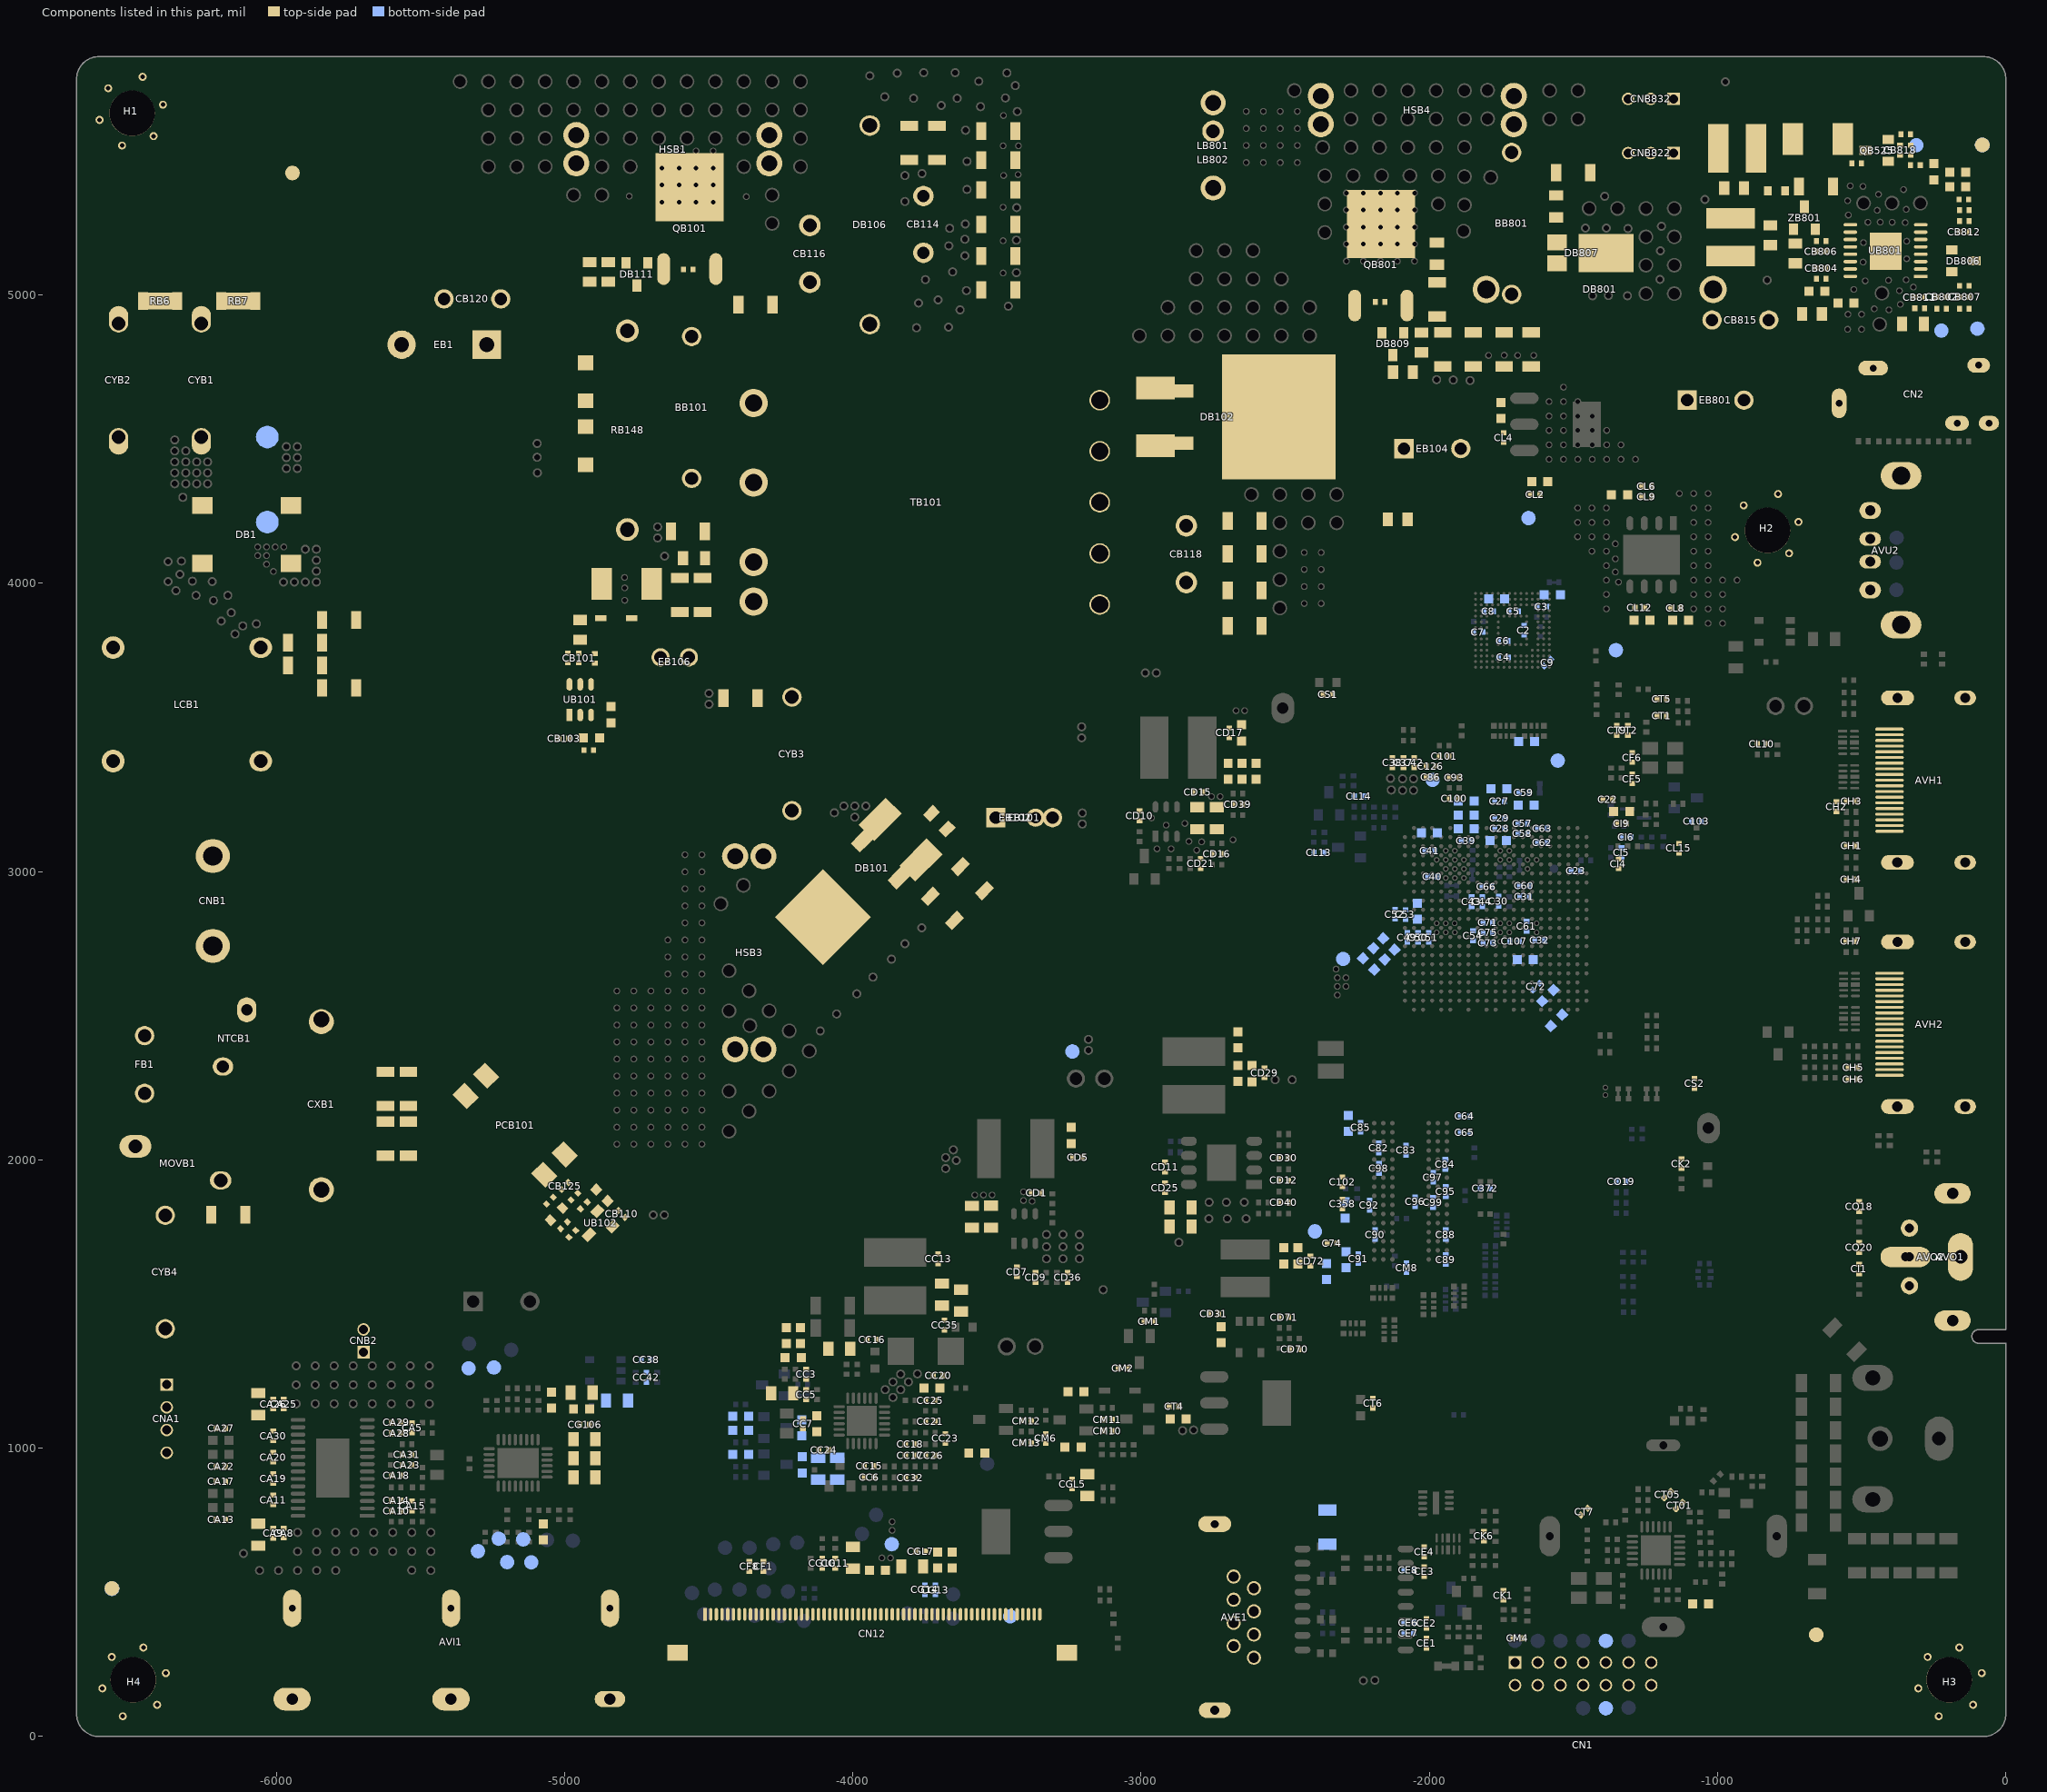
[diagram p0: the components of this part, seen from the top]
# Altium PCB MISC84395.PcbDoc (part 2 of 26)
Units mil, origin at the board's own origin, x right, y up, seen from the top; angles counter-clockwise.
Board outline 6692.91 x 5826.77 mil, 2 copper layers (TopLayer, BottomLayer), stack 61.855 mil thick; 951 components, 565 nets, 4374 pads, 1804 vias.
Unrouted connection lines stored in the file: 1.

## Classes and differential pairs (continued)
component class PS#01_XXXXXXXXXXXXXXXX: ADIM BB101 BB801 BL_ON CB101 CB102 CB103 CB109 CB110 CB111 CB113 CB114 CB116 CB117 CB118 CB120 CB125 CB802 CB803 CB804 CB805 CB806 CB807 CB809 CB810 CB811 CB812 CB813 CB814 CB815 CB816 CB818 CB819 CNB1 CNB2 CNB822 CNB832 "Conformal Coating" CXB1 CXB2 CYB1 CYB2 CYB3 CYB4 DB1 DB101 DB102 DB104 DB106 DB109 DB110 DB111 DB121 DB801 DB802 DB806 DB807 DB809 EB1 EB101 EB102 EB104 EB106 EB801 EVA1 EVA2 EVA3 EVA4 EVA5 EVA6 FB1 GD1 GD2 GD3 GD4 GL1 GL2 HSB1 HSB3 HSB4 LB801 LB802 LB804 LB805 LCB1 LCB2 ML1 MOVB1 NTCB1 PCB101 PWM_DIM QB101 QB525 QB801 RB1 RB2 RB3 RB4 RB5 RB6 RB7 RB101 RB102 RB103 RB104 RB105 RB106 RB107 RB109 RB114 RB115 RB116 RB117 RB118 RB119 RB121 RB124 RB125 RB126 RB128 RB129 RB130 RB131 RB132 RB133 RB134 RB135 RB136 RB140 RB141 RB142 RB148 RB151 RB152 RB153 RB154 RB155 RB156 RB158 RB801 RB802 RB803 RB804 RB805 RB806 RB807 RB808 RB809 RB810 RB811 RB812 RB814 RB816 RB818 RB819 RB820 RB821 RB822 RB824 RB825 RB826 RB827 RB830 RB832 RB833 RB834 RB837 TB101 TP-TDT UB101 UB102 UB801 ZB801
component class PCB_info: AI_V CAUTION COLD CQC H1 H2 H3 H4 "High Voltage" HOT M1 M2 M3 M4 M5 M6 MAC Manufacture_Info S/N1 S/N2
polygon class Poly_5mil: 5 5mil
pad class HS60: Free-HS60
pad class VIA5: Free-VIA5

## Components (designator, comment, footprint, x,y, rotation, side; value= is the part's Value field where it differs from the comment)
1V8_M "TEST" TP#1 -1554.58,3384.95 r270 bottom
3V3_M "TEST" TP#1 -1352.83,3768 r180 bottom
3V3_STB "TEST" TP#1 -1656,4226 r90 bottom
5V_STB "TEST" TP#2 -3238.17,2376 r90 bottom
5V_WIFI "TEST" TP#2 -1387.74,98 r90 bottom
+1.5V_DDR "TEST" TP#1 -2397,1752 r90 bottom
+1.05V_VDDC_CPU "TEST" TP#1 -2299,2697 r270 bottom
+1.10V_VDDC "TEST" TP#1 -1989,3318 r270 bottom
ADIM "NC/TEST" TP_BL -311,5519 r270 bottom
AI_V "AI_GRIPPER_V" AI_GRIPPER_V 6418,1068.5 r90 top
AVDD "TEST" TP#1 -3865,667 r0 bottom
AVE1 "Network terminal,DIP,RJ170-F08M1BY-B,YUQIU" RJ45-VD-16 -2803.54,414.17 r90 top locked
AVH1 "HDMI terminal,HDMI Jack,H,SMD,161031041(hull-SPCC ),VAST" HDMI-HS-1 39.37,3316.93 r90 top locked
AVH2 "HDMI terminal,HDMI Jack,H,SMD,161031041(hull-SPCC ),VAST" HDMI-HS-1 39.37,2470.47 r90 top locked
AVI1 "RCA terminal,RCA Jack,AV3,V,Yellow, White, Red,D14,DIP,RCA-339H-EP-01,CS" AV3-V14-1 -5393.7,334.65 r0 top locked
AVO1 "RCA terminal,RCA Jack,AV1,H,Orange,CH6.5,Seal,DIP,RCA-105M-EP-07-S,CS" AV1-H-1 0,1663.39 r90 top locked
AVO2 "Optical fiber terminal,OPTICAL,H,DIP,DQT-026D-2,DQ" OPTICAL-HD-3 0,1663.39 r90 top locked
AVU2 "USB terminal,USB Jack,H,Single,flange,DIP,WLUS-050F USB,WLCO" USB1-HD-2 39.37,4114.17 r90 top locked
BB101 "Ferrite bead,BEAD,70ohm Min,φ3.5×6.0×0.65mm,DIP,TP,RH3.5×6×0.8-T-LF,DL" LB/3.5*6*12.5#1 -4559,4609.68 r270 top
BB801 "Ferrite bead,BEAD,70ohm Min,φ3.5×6.0×0.65mm,DIP,TP,RH3.5×6×0.8-T-LF,DL" LB/3.5*6*12.5#2 -1714.6,5248 r270 top
BL_ON "NC/TEST" TP_BL -224,4876 r0 bottom
BT_RST "TEST" TP#2 -1387.74,332 r90 bottom
C1 "10uF-0603-X5R-±20%-6.3V" C0603 -1573.65,3960.74 r180 bottom
C2 "1uF-0402-X5R-±20%-6.3V" C0402#1 -1671.48,3836.72 r270 bottom
C3 "0.1uF-0402-X5R-±20%-16V" C0402#1 -1610.65,3918.74 r180 bottom
C4 "0.1uF-0402-X5R-±20%-16V" C0402#1 -1743.38,3742.74 r0 bottom
C5 "1uF-0402-X5R-±20%-6.3V" C0402#1 -1707.65,3902.74 r180 bottom
C6 "0.1uF-0402-X5R-±20%-16V" C0402#1 -1744.21,3799.84 r0 bottom
C7 "0.1uF-0402-X5R-±20%-16V" C0402#1 -1830.65,3830.74 r0 bottom
C8 "0.1uF-0402-X5R-±20%-16V" C0402#1 -1794.65,3902.74 r0 bottom
C9 "2.2uF-0402-X5R-±20%-6.3V" C0402#1 -1590,3724 r225 bottom
C21 "10uF-0603-X5R-±20%-6.3V" C0603 -1332.77,3208.74 r180 top
C22 "0.1uF-0402-X5R-±20%-16V" C0402#1 -1380.77,3250.74 r180 top
C23 "0.047uF-0402-X7R-±10%-16V" C0402#1 -1491.65,3002.74 r0 bottom
C25 "10uF-0603-X5R-±20%-6.3V" C0603 -1761,3107 r0 bottom
C26 "NC/10uF-0603-X5R-±20%-6.3V" C0603 -1758.97,3287.08 r0 bottom
C27 "0.1uF-0402-X7R-±10%-16V" C0402#1 -1756.47,3243.08 r0 bottom
C28 "0.1uF-0402-X7R-±10%-16V" C0402#1 -1756,3149 r0 bottom
C29 "0.1uF-0402-X7R-±10%-16V" C0402#1 -1756,3185 r0 bottom
C30 "0.1uF-0402-X7R-±10%-16V" C0402#1 -1759.66,2897.23 r90 bottom
C31 "0.1uF-0402-X7R-±10%-16V" C0402#1 -1670.01,2913.34 r180 bottom
C32 "0.1uF-0402-X7R-±10%-16V" C0402#1 -1617.44,2761.28 r180 bottom
C33 "10uF-0603-X5R-±20%-6.3V" C0603 -2000,3134 r0 bottom
C34 "Ceramic capacitor,CAP MC,6.3V,22uF,±20%,X5R,0603,SMD,TP" C0603 -1872.67,3244.15 r180 bottom
C35 "Ceramic capacitor,CAP MC,6.3V,22uF,±20%,X5R,0603,SMD,TP" C0603 -1872.67,3148.15 r180 bottom
C36 "NC/Ceramic capacitor,CAP MC,6.3V,22uF,±20%,X5R,0603,SMD,TP" C0603 -1872.67,3195.15 r180 bottom
C37 "0.1uF-0402-X7R-±10%-16V" C0402#1 -2090.06,3378.06 r270 top
C38 "NC/0.1uF-0402-X5R-±20%-16V" C0402#1 -2128.06,3378.06 r270 top
C39 "NC/0.1uF-0402-X5R-±20%-16V" C0402#1 -1872,3107 r180 bottom
C40 "0.1uF-0402-X7R-±10%-16V" C0402#1 -1989,2982 r0 bottom
C41 "0.1uF-0402-X7R-±10%-16V" C0402#1 -1998,3072 r0 bottom
C42 "0.1uF-0402-X7R-±10%-16V" C0402#1 -2053.06,3378.06 r270 top
C43 "0.1uF-0402-X7R-±10%-16V" C0402#1 -1853.65,2895.74 r90 bottom
C44 "1uF-0402-X5R-±20%-6.3V" C0402#1 -1816.65,2895.74 r90 bottom
C45 "NC/10uF-0603-X5R-±20%-6.3V" C0603 -2042,2863 r270 bottom
C46 "10uF-0603-X5R-±20%-6.3V" C0603 -2174.67,2714.51 r135 bottom
C47 "NC/10uF-0603-X5R-±20%-6.3V" C0603 -2210.67,2679.51 r135 bottom
C48 "10uF-0603-X5R-±20%-6.3V" C0603 -2140.52,2748.74 r135 bottom
C49 "NC/0.1uF-0402-X7R-±10%-16V" C0402#1 -2076.48,2771.72 r90 bottom
C50 "Ceramic capacitor,CAP MC,50V,1000pF,±10%,X7R,0402,SMD,TP" C0402#1 -2039.48,2771.72 r90 bottom
C51 "0.1uF-0402-X7R-±10%-16V" C0402#1 -2002.48,2771.72 r90 bottom
C52 "NC/0.1uF-0402-X7R-±10%-16V" C0402#1 -2119,2852 r270 bottom
C53 "Ceramic capacitor,CAP MC,6.3V,0.47uF,±10%,X5R,0402,SMD,TP" C0402#1 -2083,2851 r270 bottom
C54 "1uF-0402-X5R-±20%-6.3V" C0402#1 -1848.65,2777.74 r270 bottom
C55 "10uF-0603-X5R-±20%-6.3V" C0603 -1664,3231 r180 bottom
C56 "NC/10uF-0603-X5R-±20%-6.3V" C0603 -1662.52,3451.34 r180 bottom
C57 "0.1uF-0402-X7R-±10%-16V" C0402#1 -1676.15,3166.97 r180 bottom
C58 "0.1uF-0402-X7R-±10%-16V" C0402#1 -1676.15,3132.09 r180 bottom
C59 "0.1uF-0402-X7R-±10%-16V" C0402#1 -1672,3274 r180 bottom
C60 "1uF-0402-X5R-±20%-6.3V" C0402#1 -1670.2,2950.02 r180 bottom
C61 "0.1uF-0402-X7R-±10%-16V" C0402#1 -1662.56,2810.22 r270 bottom
C62 "NC/1uF-0402-X5R-±20%-6.3V" C0402#1 -1607.65,3100.74 r180 bottom
C63 "0.1uF-0402-X7R-±10%-16V" C0402#1 -1607.65,3149.74 r180 bottom
C64 "1uF-0402-X5R-±20%-6.3V" C0402#1 -1876.27,2151.08 r0 bottom
C65 "1uF-0402-X5R-±20%-6.3V" C0402#1 -1876.27,2095.58 r180 bottom
C66 "0.1uF-0402-X7R-±10%-16V" C0402#1 -1800.65,2947.74 r0 bottom
C71 "0.1uF-0402-X7R-±10%-16V" C0402#1 -1796.65,2822.74 r0 bottom
C72 "0.1uF-0402-X7R-±10%-16V" C0402#1 -1629,2601 r225 bottom
C73 "0.1uF-0402-X7R-±10%-16V" C0402#1 -1796.65,2752.74 r0 bottom
C74 "1uF-0402-X5R-±20%-6.3V" C0402#1 -2337.5,1710.95 r180 top
C75 "1uF-0402-X5R-±20%-6.3V" C0402#1 -1796.65,2787.74 r0 bottom
C80 "10uF-0603-X5R-±20%-6.3V" C0603 -2291.71,1826.53 r90 bottom
C81 "10uF-0603-X5R-±20%-6.3V" C0603 -2357.57,1613 r90 bottom
C82 "0.1uF-0402-X5R-±20%-16V" C0402#1 -2175.48,2041.8 r270 bottom
C83 "0.1uF-0402-X5R-±20%-16V" C0402#1 -2080.99,2033.92 r270 bottom
C84 "0.1uF-0402-X5R-±20%-16V" C0402#1 -1944.97,1984.7 r90 bottom
C85 "1uF-0402-X5R-±20%-6.3V" C0402#1 -2238.47,2112.82 r270 bottom
C86 "0.01uF-0402-X7R-±10%-50V" C0402#1 -1994.65,3327.74 r180 top
C87 "10uF-0603-X5R-±20%-6.3V" C0603 -2288.48,1653.72 r90 bottom
C88 "0.1uF-0402-X5R-±20%-16V" C0402#1 -1943.47,1740.92 r90 bottom
C89 "0.1uF-0402-X5R-±20%-16V" C0402#1 -1943.2,1654.31 r90 bottom
C90 "0.1uF-0402-X5R-±20%-16V" C0402#1 -2187.97,1740.92 r90 bottom
C91 "0.1uF-0402-X5R-±20%-16V" C0402#1 -2246.48,1657.72 r90 bottom
C92 "1uF-0402-X5R-±20%-6.3V" C0402#1 -2207.47,1842.97 r90 bottom
C93 "NC/0.01uF-0402-X7R-±10%-16V" C0402#1 -1913.28,3326.48 r180 top
C94 "10uF-0603-X5R-±20%-6.3V" C0603 -2281.48,2126.72 r270 bottom
C95 "0.1uF-0402-X5R-±20%-16V" C0402#1 -1943.2,1890.22 r90 bottom
C96 "0.1uF-0402-X5R-±20%-16V" C0402#1 -2049.48,1854.72 r270 bottom
C97 "0.1uF-0402-X5R-±20%-16V" C0402#1 -1986.51,1939.43 r270 bottom
C98 "0.1uF-0402-X5R-±20%-16V" C0402#1 -2174.97,1970.62 r270 bottom
C99 "1uF-0402-X5R-±20%-6.3V" C0402#1 -1987.47,1852.51 r270 bottom
C100 "0.1uF-0402-X5R-±20%-16V" C0402#1 -1913.26,3253 r180 top
C101 "1000pF-0402-X7R-±10%-50V" C0402#1 -1948.65,3399.74 r0 top
C102 "1000pF-0402-X7R-±10%-50V" C0402#1 -2301.47,1923.69 r90 top
C103 "NC/1uF-0402-X5R-±20%-16V" C0402#1 -1073,3174 r0 bottom
C104 "10uF-0603-X5R-±20%-6.3V" C0603 -1588.83,2570 r225 bottom
C105 "10uF-0603-X5R-±20%-6.3V" C0603 -1667,2694 r180 bottom
C106 "NC/10uF-0603-X5R-±20%-6.3V" C0603 -1559.17,2483.66 r225 bottom
C107 "0.1uF-0402-X7R-±10%-16V" C0402#1 -1704.47,2758.58 r180 bottom
C108 "NC/10uF-0603-X5R-±20%-6.3V" C0603 -1766.65,3945.74 r0 bottom
C126 "NC/0.1uF-0402-X5R-±20%-16V" C0402#1 -1994.65,3365.74 r180 top
C358 "0.1uF-0402-X5R-±20%-16V" C0402#1 -2301.47,1847.22 r90 top
C372 "0.1uF-0402-X5R-±20%-16V" C0402#1 -1806.07,1901.08 r180 bottom
CA1 "10uF-0805-X5R-±20%-16V" C0805 -6061.94,700 r90 top
CA2 "NC/10uF-0805-X5R-±20%-16V" C0805 -6061.94,1153 r270 top
CA5 "3300pF-0402-X7R-±10%-50V" C0402#1 -5528.99,1070.94 r270 top
CA8 "0.22uF-0402-X5R-±10%-16V" C0402#1 -5974.23,705.53 r90 top
CA9 "NC/Ceramic capacitor,CAP MC,50V,1000pF,±10%,X7R,0402,SMD,TP" C0402#1 -6010.23,705.26 r90 top
CA10 "0.22uF-0402-X5R-±10%-16V" C0402#1 -5583.87,781.96 r0 top
CA11 "0.22uF-0402-X5R-±10%-16V" C0402#1 -6010.6,820.94 r270 top
CA13 "2200pF-0402-X7R-±10%-50V" C0402#1 -6192.01,752.06 r180 top
CA14 "0.22uF-0402-X5R-±10%-16V" C0402#1 -5583.87,818.96 r0 top
CA15 "3300pF-0402-X7R-±10%-50V" C0402#1 -5528.99,800 r270 top
CA17 "2200pF-0402-X7R-±10%-50V" C0402#1 -6192.02,885.16 r0 top
CA18 "1uF-0402-X5R-±20%-16V" C0402#1 -5583.23,906 r0 top
CA19 "0.22uF-0402-X5R-±10%-16V" C0402#1 -6010.6,894.94 r90 top
CA20 "0.22uF-0402-X5R-±10%-16V" C0402#1 -6010.6,968.94 r270 top
CA22 "2200pF-0402-X7R-±10%-50V" C0402#1 -6192.02,937.06 r180 top
CA23 "1uF-0402-X5R-±20%-16V" C0402#1 -5546.6,941.94 r0 top
CA25 "0.22uF-0402-X5R-±10%-16V" C0402#1 -5974.17,1153.23 r90 top
CA26 "NC/Ceramic capacitor,CAP MC,50V,1000pF,±10%,X7R,0402,SMD,TP" C0402#1 -6010.53,1153.25 r270 top
CA27 "2200pF-0402-X7R-±10%-50V" C0402#1 -6192.08,1069 r0 top
CA28 "0.22uF-0402-X5R-±10%-16V" C0402#1 -5583.87,1051.94 r0 top
CA29 "0.22uF-0402-X5R-±10%-16V" C0402#1 -5583.87,1088.94 r0 top
CA30 "0.22uF-0402-X5R-±10%-16V" C0402#1 -6010.6,1042.94 r90 top
CA31 "NC/1uF-0402-X5R-±20%-16V" C0402#1 -5546.6,977.94 r0 top
CAUTION "CAUTION" CAUTION -5864.96,2965.25 r90 bottom
CB101 "100pF-0402-NPO-±5%-50V" C0402#1 -4950.43,3740.81 r90 top
CB102 "0.1uF-0603-X7R-±10%-50V" C0603 -4838.49,3544.11 r270 top
CB103 "1000pF-0402-X7R-±10%-50V" C0402#1 -5002.22,3461.3 r180 top
CB109 "Ceramic capacitor,CAP MC,25V,0.22uF,±10%,X7R,0603,SMD,TP" C0603 -4870.33,1877.33 r135 top
CB110 "NC/1000pF-0402-X7R-±10%-50V" C0402#1 -4801.34,1812.34 r315 top
CB111 "Ceramic capacitor,CAP MC,50V,220pF,±5%,NPO,0603,SMD,TP" C0603 -4906.49,3464.3 r180 top
CB113 "NC/220PF-0805-NPO-±10%-200V" C0805 -4551,4086.3 r180 top
CB114 "Film capacitor,CAP PE,400V,4700pF,±10%,P,5.0mm,PC,DIP,TP,KEMET" CAP8*2.5-V-5 -3755,5244.57 r270 top
CB116 "Ceramic capacitor,CAP CD,2KV,100pF,±5%,SL,IK,5.0mm,DIP,TP,Walsin" CAP6.5*5-V-5-1 -4149,5142.57 r90 top
CB117 "1000pF-0805-NPO-±10%-200V" C0805 -3699.89,3174.89 r315 top
CB118 "Ceramic capacitor,CAP CD,1KV,1000pF,±10%,Y5R,IK,5.0mm,DIP,TP,Walsin" CAP8.5*5-V-5 -2843,4101 r270 top
CB120 "NC/Ceramic capacitor,CAP CD,1KV,4700pF,±20%,Y5U,K,5.0mm,DIP,TP,Walsin" CAP10*4.5-V-5 -5319.57,4986 r0 top
CB125 "NC/Ceramic capacitor,CAP MC,50V,0.022uF,±10%,X7R,0402,SMD,TP" C0402#1 -4999.41,1909.71 r225 top
CB802 "220pF-0402-NPO-±5%-50V" C0402#1 -223,4992.32 r180 top
CB803 "0.1uF-0603-X7R-±10%-50V" C0603 -555.19,4971 r180 top
CB804 "220pF-0402-NPO-±5%-50V" C0402#1 -640.74,5091.94 r0 top
CB805 "0.47uF-0805-X7R-±10%-50V" C0805 -322.3,4899.32 r0 top
CB806 "1000pF-0402-X7R-±10%-50V" C0402#1 -640.77,5150.88 r0 top
CB807 "220pF-0402-NPO-±5%-50V" C0402#1 -144.27,4992.31 r0 top
CB809 "220PF-0805-NPO-±10%-200V" C0805 -1974,5143.03 r90 top
CB810 "220PF-0805-NPO-±10%-200V" C0805 -1560,5307 r270 top
CB811 "NC/1000pF-0402-X7R-±10%-50V" C0402#1 -299.23,4992.18 r180 top
CB812 "NC/1000pF-0402-X7R-±10%-50V" C0402#1 -144.69,5218 r0 top
CB813 "0.1uF-0603-X7R-±10%-50V" C0603 -656,5013 r0 top
CB814 "Ceramic capacitor,CAP MC,25V,1uF,±10%,X7R,0603,SMD,TP" C0603 -166.81,5425 r180 top
CB815 "NC/CK45-B3AD102KYPNX(TDK)" CAP7.5*2.5-V-5 -921,4913 r0 top
CB816 "NC/Ceramic capacitor,CAP MC,25V,1uF,±10%,X7R,0603,SMD,TP" C0603 -166.81,5375 r180 top
CB818 "NC/1000pF-0402-X7R-±10%-50V" C0402#1 -367,5502.26 r90 top
CB819 "NC/Ceramic capacitor,CAP MC,25V,1uF,±10%,X7R,0603,SMD,TP" C0603 -250,5427 r270 top
CC1 "NC/Ceramic capacitor,CAP MC,25V,10uF,±10%,X5R,0805,SMD,TP" C0805 -4000,620 r270 top
CC2 "Ceramic capacitor,CAP MC,25V,10uF,±10%,X5R,0805,SMD,TP" C0805 -4245.03,1191 r0 top
CC3 "NC/0.1uF-0402-X5R-±20%-16V" C0402#1 -4162.24,1256.84 r90 top
CC4 "Ceramic capacitor,CAP MC,25V,1uF,±10%,X5R,0603,SMD,TP" C0603 -4125,1085 r90 top
CC5 "NC/1uF-0402-X5R-±20%-16V" C0402#1 -4162,1186 r270 top
CC6 "NC/NC/1uF-0402-X5R-±20%-6.3V" C0402#1 -3943.15,899 r180 top
CC7 "Ceramic capacitor,CAP MC,25V,0.1uF,±20%,X5R,0402,SMD,TP" C0402#1 -4173,1085 r270 top
CC8 "10uF-0805-X5R-±20%-16V" C0805 -3691,1533 r270 top
CC9 "NC/0.1uF-0603-X7R-±10%-50V" C0603 -4231,1391 r90 top
CC10 "0.1uF-0603-X7R-±10%-50V" C0603 -4181,1391 r90 top
CC11 "0.1uF-0603-X7R-±10%-50V" C0603 -4206.81,1314 r180 top
CC12 "NC/10uF-0805-X5R-±20%-16V" C0805 -3624,1512.03 r270 top
CC13 "NC/0.1uF-0402-X5R-±20%-16V" C0402#1 -3704,1657 r270 top
CC14 "NC/?" C0805 -4047.03,1345 r0 top
CC15 "1uF-0402-X5R-±20%-6.3V" C0402#1 -3943,938 r0 top
CC16 "Ceramic capacitor,CAP MC,50V,33pF,±5%,NPO,0402,SMD,TP" C0402#1 -3934,1377 r0 top
CC17 "1uF-0402-X5R-±20%-6.3V" C0402#1 -3801,975 r180 top
CC18 "1uF-0402-X5R-±20%-6.3V" C0402#1 -3801,1014 r0 top
CC19 "NC/Ceramic capacitor,CAP MC,25V,10uF,±10%,X5R,0805,SMD,TP" C0805 -3794,590 r0 top
CC20 "Ceramic capacitor,CAP MC,25V,0.1uF,±20%,X5R,0402,SMD,TP" C0402#1 -3704,1252 r0 top
CC21 "Ceramic capacitor,CAP MC,50V,1000pF,±10%,X7R,0402,SMD,TP" C0402#1 -3731,1093 r0 top
CC22 "NC/1uF-0603-X5R-±10%-50V" C0603 -3725.81,1209 r180 top
CC23 "NC/0.1uF-0402-X5R-±20%-16V" C0402#1 -3679,1033.74 r270 top
CC24 "0.1uF-0402-X5R-±20%-16V" C0402#1 -4100.84,994 r180 top
CC25 "NC/33pF-0402-NPO-±5%-50V" C0402#1 -3731,1166 r0 top
CC26 "NC/33pF-0402-NPO-±5%-50V" C0402#1 -3731,975 r0 top
CC27 "0.1uF-0603-X7R-±10%-50V" C0603 -4176,942.19 r90 bottom
CC28 "1uF-0603-X5R-±10%-50V" C0603 -4389,978.19 r180 bottom
CC29 "10uF-0805-X5R-±20%-16V" C0805 -4120.05,929.03 r90 bottom
CC30 "NC/10uF-0805-X5R-±20%-16V" C0805 -4054,929.03 r90 bottom
CC31 "NC/0.1uF-0603-X7R-±10%-50V" C0603 -4177,1070.19 r270 bottom
CC32 "NC/33pF-0402-NPO-±5%-50V" C0402#1 -3801,898 r0 top
CC33 "1uF-0603-X5R-±10%-50V" C0603 -4389,1110.19 r0 bottom
CC34 "0.1uF-0603-X7R-±10%-50V" C0603 -4389,1062.19 r0 bottom
CC35 "Ceramic capacitor,CAP MC,50V,33pF,±5%,NPO,0402,SMD,TP" C0402#1 -3682,1427 r90 top
CC36 "Ceramic capacitor,CAP MC,25V,1uF,±10%,X5R,0603,SMD,TP" C0603 -5073,710 r270 top
CC38 "0.1uF-0402-X5R-±20%-16V" C0402#1 -4717,1306.73 r0 bottom
CC42 "0.1uF-0402-X5R-±20%-16V" C0402#1 -4716,1245.73 r90 bottom
CC43 "10uF-0805-X5R-±20%-16V" C0805 -4818,1164.73 r180 bottom
CD1 "NC/0.1uF-0402-X5R-±20%-16V" C0402#1 -3363.15,1885 r180 top
CD2 "NC/10uF-0603-X5R-±20%-6.3V" C0603 -2664,2416 r270 top
CD4 "10uF-0805-X5R-±20%-16V" C0805 -3586.86,1802.89 r270 top
CD5 "NC/0.1uF-0402-X7R-±10%-16V" C0402#1 -3220.15,2008 r180 top
CD6 "NC/10uF-0805-X5R-±20%-16V" C0805 -3521,1803 r270 top
CD7 "0.1uF-0402-X5R-±20%-16V" C0402#1 -3431,1612 r270 top
CD8 "10uF-0603-X5R-±20%-10V" C0603 -3242,2085 r90 top
CD9 "NC/10pF-0402-NPO-±5%-50V" C0402#1 -3366,1592.27 r270 top
CD10 "0.1uF-0402-X5R-±20%-16V" C0402#1 -3005,3193.33 r90 top
CD11 "0.1uF-0402-X5R-±20%-16V" C0402#1 -2917,1975 r270 top
CD12 "330pF-0402-NPO-±5%-50V" C0402#1 -2505,1929 r0 top
CD13 "NC/10uF-0805-X5R-±20%-16V" C0805 -2737,3185.19 r270 top
CD14 "10uF-0805-X5R-±20%-16V" C0805 -2805,3185.19 r270 top
CD15 "NC/0.1uF-0402-X5R-±20%-16V" C0402#1 -2803,3276 r0 top
CD16 "NC/NC/56pF-0402-NPO-±5%-50V" C0402#1 -2736.91,3060.93 r0 top
CD17 "NC/0.1uF-0402-X5R-±20%-16V" C0402#1 -2694,3481.03 r90 top
CD18 "NC/10uF-0603-X5R-±20%-6.3V" C0603 -2650,3348.19 r270 top
CD19 "10uF-0603-X5R-±20%-6.3V" C0603 -2698,3348.19 r270 top
CD20 "NC/10uF-0603-X5R-±20%-6.3V" C0603 -2651,3481.19 r90 top
CD21 "NC/8pF-0402-NPO-±5%-50V" C0402#1 -2793.26,3027.71 r270 top
CD23 "NC/10uF-0805-X5R-±20%-16V" C0805 -2862.97,1769 r180 top
CD24 "10uF-0805-X5R-±20%-16V" C0805 -2863,1835 r180 top
CD25 "NC/0.1uF-0402-X5R-±20%-16V" C0402#1 -2917,1903.16 r270 top
CD26 "10uF-0603-X5R-±20%-6.3V" C0603 -2664.08,2300.12 r90 top
CD28 "10uF-0603-X5R-±20%-6.3V" C0603 -2615.08,2299.12 r90 top
CD29 "NC/0.1uF-0402-X5R-±20%-16V" C0402#1 -2572,2302 r270 top
CD30 "1uF-0402-X5R-±20%-6.3V" C0402#1 -2506,2006 r0 top
CD31 "NC/0.1uF-0402-X7R-±10%-16V" C0402#1 -2748,1466 r180 top
CD36 "220pF-0402-NPO-±5%-50V" C0402#1 -3255,1592.27 r270 top
CD39 "0.1uF-0402-X5R-±20%-16V" C0402#1 -2664.29,3232.87 r0 top
CD40 "0.1uF-0402-X5R-±20%-16V" C0402#1 -2505,1852 r0 top
CD45 "10uF-0603-X5R-±20%-6.3V" C0603 -2601,3348 r270 top
CD69 "10uF-0603-X5R-±20%-10V" C0603 -2722,1393.81 r270 top
CD70 "Ceramic capacitor,CAP MC,50V,68pF,±5%,NPO,0402,SMD,TP" C0402#1 -2467.74,1343.26 r0 top
CD71 "NC/0.1uF-0402-X5R-±20%-16V" C0402#1 -2504.73,1454.26 r180 top
CD72 "NC/0.1uF-0402-X5R-±20%-16V" C0402#1 -2413,1649.1 r90 top
CD73 "10uF-0603-X5R-±20%-6.3V" C0603 -2456,1667.26 r270 top
CD74 "10uF-0603-X5R-±20%-6.3V" C0603 -2505,1667.26 r270 top
CE1 "NC/7pF-0402-NPO-±5%-50V" C0402#1 -2010.1,323.71 r90 top
CE2 "NC/7pF-0402-NPO-±5%-50V" C0402#1 -2010.1,392.71 r270 top
CE3 "NC/7pF-0402-NPO-±5%-50V" C0402#1 -2018,572 r90 top
CE4 "NC/7pF-0402-NPO-±5%-50V" C0402#1 -2018,640.85 r270 top
CE5 "0ohm-1206-±5%-1/4W" C1206 -2354,726 r90 bottom
CE6 "NC/0.1uF-0402-X5R-±20%-16V" C0402#1 -2071.94,394.94 r180 bottom
CE7 "NC/0.01uF-0402-X7R-±10%-16V" C0402#1 -2071.94,358.94 r180 bottom
CE8 "NC/0.1uF-0402-X5R-±20%-16V" C0402#1 -2072,577 r0 bottom
CF1 "NC/NC/5pF-0402-NPO-±5%-50V" C0402#1 -4310,590 r270 top
CF5 "Ceramic capacitor,CAP MC,50V,15pF,±5%,NPO,0402,SMD,TP" C0402#1 -1296.65,3321.74 r270 top
CF6 "Ceramic capacitor,CAP MC,50V,15pF,±5%,NPO,0402,SMD,TP" C0402#1 -1296.65,3395.74 r90 top
CF8 "NC/NC/5pF-0402-NPO-±5%-50V" C0402#1 -4359,589.85 r270 top
CG1 "10uF-0805-X5R-±20%-16V" C0805 -4931,965 r0 top
CG2 "10uF-0805-X5R-±20%-16V" C0805 -4931,1031 r0 top
CG3 "10uF-0805-X5R-±20%-16V" C0805 -4931,899 r0 top
CG10 "NC/0.1uF-0402-X7R-±10%-16V" C0402#1 -4106,601 r90 top
CG11 "NC/0.1uF-0402-X7R-±10%-16V" C0402#1 -4061,601 r90 top
CG12 "NC/1uF-0603-X5R-±10%-25V" C0603 -3915,577 r180 top
CG13 "NC/0.1uF-0402-X7R-±10%-16V" C0402#1 -3714,508.74 r270 bottom
CG14 "NC/0.1uF-0402-X7R-±10%-16V" C0402#1 -3750,509 r270 bottom
CG103 "1uF-0603-X5R-±10%-50V" C0603 -5045,1167 r270 top
CG104 "Ceramic capacitor,CAP MC,50V,4.7uF,±20%,X5R,0805,SMD,TP" C0805 -4940.97,1193 r0 top
CG105 "1uF-0603-X5R-±10%-50V" C0603 -4940.97,1136 r180 top
CG106 "NC/0.1uF-0402-X7R-±10%-16V" C0402#1 -4930,1082 r180 top
CGL4 "NC/10uF-0805-X5R-±20%-16V" C0805 -3187,872 r270 top
CGL5 "NC/0.1uF-0402-X7R-±10%-16V" C0402#1 -3239,876 r90 top
CGL6 "NC/10uF-0603-X5R-±20%-6.3V" C0603 -3705,612 r270 top
CGL7 "NC/0.1uF-0402-X7R-±10%-16V" C0402#1 -3764.84,642 r180 top
CGL49 "10uF-0603-X5R-±20%-6.3V" C0603 -3656,612 r270 top
CH1 "NC/1000pF-0402-X7R-±10%-50V" C0402#1 -536.38,3088.99 r0 top
CH2 "1uF-0402-X5R-±20%-6.3V" C0402#1 -587.83,3225 r270 top
CH3 "NC/22pF-0402-NPO-±5%-50V" C0402#1 -536.64,3244.29 r180 top
CH4 "NC/1000pF-0402-X7R-±10%-50V" C0402#1 -536.84,2973 r0 top
CH5 "NC/1000pF-0402-X7R-±10%-50V" C0402#1 -530.37,2319.87 r0 top
CH6 "NC/1000pF-0402-X7R-±10%-50V" C0402#1 -530.37,2279.87 r180 top
CH7 "NC/22pF-0402-NPO-±5%-50V" C0402#1 -537.37,2758.16 r0 top
CI1 "NC/0.1uF-0402-X5R-±20%-16V" C0402#1 -509.01,1621.7 r90 top
CI4 "0.047uF-0402-X7R-±10%-16V" C0402#1 -1343.65,3026.74 r90 top
CI5 "56pF-0402-NPO-±5%-50V" C0402#1 -1333.65,3065.47 r270 bottom
CI6 "1uF-0402-X5R-±20%-6.3V" C0402#1 -1317.65,3119.74 r180 bottom
CI9 "1uF-0402-X5R-±20%-6.3V" C0402#1 -1333.5,3166.74 r180 top
CK1 "1000pF-0402-X7R-±10%-50V" C0402#1 -1743,490 r90 top
CK2 "0.01uF-0402-X7R-±10%-50V" C0402#1 -1125,1986.88 r90 top
CK6 "33pF-0402-NPO-±5%-50V" C0402#1 -1811,695 r90 top
CL1 "NC/10uF-0603-X5R-±20%-10V" C0603 -1617,4352 r180 top
CL2 "0.1uF-0402-X5R-±20%-16V" C0402#1 -1633,4308 r0 top
CL3 "NC/10uF-0603-X5R-±20%-6.3V" C0603 -1752,4599 r90 top
CL4 "1uF-0402-X5R-±20%-6.3V" C0402#1 -1742,4505 r270 top
CL5 "NC/10uF-0603-X5R-±20%-10V" C0603 -1340.37,4306 r0 top
CL6 "0.1uF-0402-X7R-±10%-16V" C0402#1 -1246.37,4336 r180 top
CL7 "NC/10uF-0603-X5R-±20%-6.3V" C0603 -1128.02,3871.83 r180 top
CL8 "1uF-0402-X5R-±20%-6.3V" C0402#1 -1146.02,3913.83 r180 top
CL9 "0.1uF-0402-X7R-±10%-16V" C0402#1 -1246.37,4300 r180 top
CL10 "NC/0.1uF-0402-X5R-±20%-16V" C0402#1 -845.83,3443 r180 top
CL11 "NC/10uF-0603-X5R-±20%-6.3V" C0603 -1262.2,3872 r0 top
CL12 "1uF-0402-X5R-±20%-6.3V" C0402#1 -1270.2,3915 r0 top
CL13 "NC/0.1uF-0402-X5R-±20%-16V" C0402#1 -2383,3066 r0 bottom
CL14 "NC/0.1uF-0402-X5R-±20%-16V" C0402#1 -2244,3261 r180 bottom
CL15 "NC/0.1uF-0402-X5R-±20%-16V" C0402#1 -1134,3081 r270 top
CLK1 "TEST" TP#2 -5300.26,643 r270 bottom
CLK2 "TEST" TP#2 -5228.26,686 r180 bottom
CLK3 "TEST" TP#2 -5199.26,605 r180 bottom
CLK4 "TEST" TP#2 -5143.26,684 r180 bottom
CLK5 "TEST" TP#1 -3454,417 r270 bottom
CLK6 "TEST" TP#2 -5115.26,604 r180 bottom
CM1 "0.1uF-0402-X5R-±20%-16V" C0402#1 -2972,1440 r0 top
CM2 "NC/0.1uF-0402-X5R-±20%-16V" C0402#1 -3063,1277 r180 top
CM3 "NC/10uF-0603-X5R-±20%-10V" C0603 -3226,1196 r0 top
CM4 "0.01uF-0402-X7R-±10%-50V" C0402#1 -1693.73,341 r180 top
CM6 "NC/0.1uF-0402-X5R-±20%-16V" C0402#1 -3331,1034 r270 top
CM7 "NC/10uF-0603-X5R-±20%-6.3V" C0603 -3236,1004 r180 top
CM8 "0.01uF-0402-X7R-±10%-50V" C0402#1 -2079.47,1625.85 r270 bottom
CM9 "NC/10uF-0603-X5R-±20%-6.3V" C0603 -3570,984 r0 top
CM10 "NC/0.022uF-0402-X7R-±10%-50V" C0402#1 -3117,1060 r180 top
CM11 "Ceramic capacitor,CAP MC,16V,0.22uF,±20%,X5R,0402,SMD,TP" C0402#1 -3117,1099 r180 top
CM12 "Ceramic capacitor,CAP MC,16V,0.22uF,±20%,X5R,0402,SMD,TP" C0402#1 -3398,1095 r180 top
CM13 "NC/0.022uF-0402-X7R-±10%-50V" C0402#1 -3398,1018 r0 top
CN1 "Connector socket,connect jack,2×7Pin,D2.0,L,Fool-proofing,Black,L=2.5mm,DIP,JN-2.0-2×7PW-H=5.6-PC=2.5,XFE" SIP2*7H/2.0DM-8 -1466.54,-92.69 r0 top locked
CN2 "Earphone jack,H,Φ3.5,CH2.5,Black,switch,DIP,PJ-304L-EP,CS" PHONE-HD-54 0,4655.51 r90 top locked
CN12 "FFC socket,FFC connector,60Pin,D0.5,Bottom,lock,SMD,CAAAR060A,FOOSUNG" FFC60H/0.5S-13 -3932.01,357.17 r0 top locked
CNA1 "Connector socket,connect jack,4Pin,D2.0,L,STEP,Fool-proofing,Nature,L=2.8,DIP,W2011-04RVA-SN1-ENSY,XYDT" SIP4H/2.0D-6 -6380,1102.36 r270 top locked
CNB1 "Connector socket,connect jack,2Pin,D7.92,L,SNAP,Fool-proofing,Nature,L=2.8mm,DIP,W7913-02RVA-S39SY,XYDT" CON2-H7.92 -6220,2898 r0 top locked
CNB2 "Connector socket,connect jack,2Pin,D2.0,D,Beige,L=2.8mm,DIP,W2011-02SVA-SN8-ENSY,XYDT" SIP2/2.0D-1 -5696.94,1372.63 r90 top
CNB822 "Connector socket,connect jack,3Pin,D2.0,L,SNAP,STEP,Fool-proofing,nature,L=2.8mm,DIP,CNJST" SIP3H/2.0D-3 -1231.74,5492 r180 top
CNB832 "NC/Connector socket,connect jack,3Pin,D2.0,D,L=2.8mm,DIP,AMA" SIP3/2.0D-CP -1232,5680 r180 top
CO18 "0.1uF-0402-X7R-±10%-16V" C0402#1 -508.99,1838.27 r270 top
CO19 "33pF-0402-NPO-±5%-50V" C0402#1 -1334.74,1925.06 r0 bottom
CO20 "330pF-0402-NPO-±5%-50V" C0402#1 -508.99,1696.27 r270 top
COLD "COLD" COLD -3385.17,3572.3 r0 top
"Conformal Coating" "NC/Conformal coating,25kg/Can,Peters" "Conformal Coating" -5648,3807 r270 top
CPV1 "TEST" TP#2 -5245,1280 r180 bottom
CPV2 "TEST" TP#2 -5333,1277 r180 bottom
CQC "CQC" CQC -3192,433 r270 top
CS1 "Ceramic capacitor,CAP MC,50V,22pF,±5%,NPO,0402,SMD,TP" C0402#1 -2352,3614 r0 top
CS2 "Ceramic capacitor,CAP MC,50V,22pF,±5%,NPO,0402,SMD,TP" C0402#1 -1080,2265 r90 top
CT01 "NC/33pF-0402-NPO-±5%-50V" C0402#2 -1133,801 r225 top
CT1 "33pF-0402-NPO-±5%-50V" C0402#1 -1194.15,3540 r180 top
CT2 "0.1uF-0402-X5R-±20%-16V" C0402#1 -1311.65,3489.74 r270 top
CT3 "NC/10uF-0603-X5R-±20%-6.3V" C0603 -2871,1102 r0 top
CT4 "NC/0.1uF-0402-X5R-±20%-16V" C0402#1 -2886.26,1145 r180 top
CT05 "NC/33pF-0402-NPO-±5%-50V" C0402#2 -1174,839 r225 top
CT5 "33pF-0402-NPO-±5%-50V" C0402#1 -1194,3598 r0 top
CT6 "NC/0.1uF-0402-X5R-±20%-16V" C0402#1 -2196,1156 r90 top
CT7 "0.1uF-0402-X5R-±20%-16V" C0402#1 -1462.04,779.96 r225 top
CT8 "10uF-0603-X5R-±20%-6.3V" C0603 -1059,460 r0 top
CT9 "0.1uF-0402-X5R-±20%-16V" C0402#1 -1349.65,3489.74 r270 top